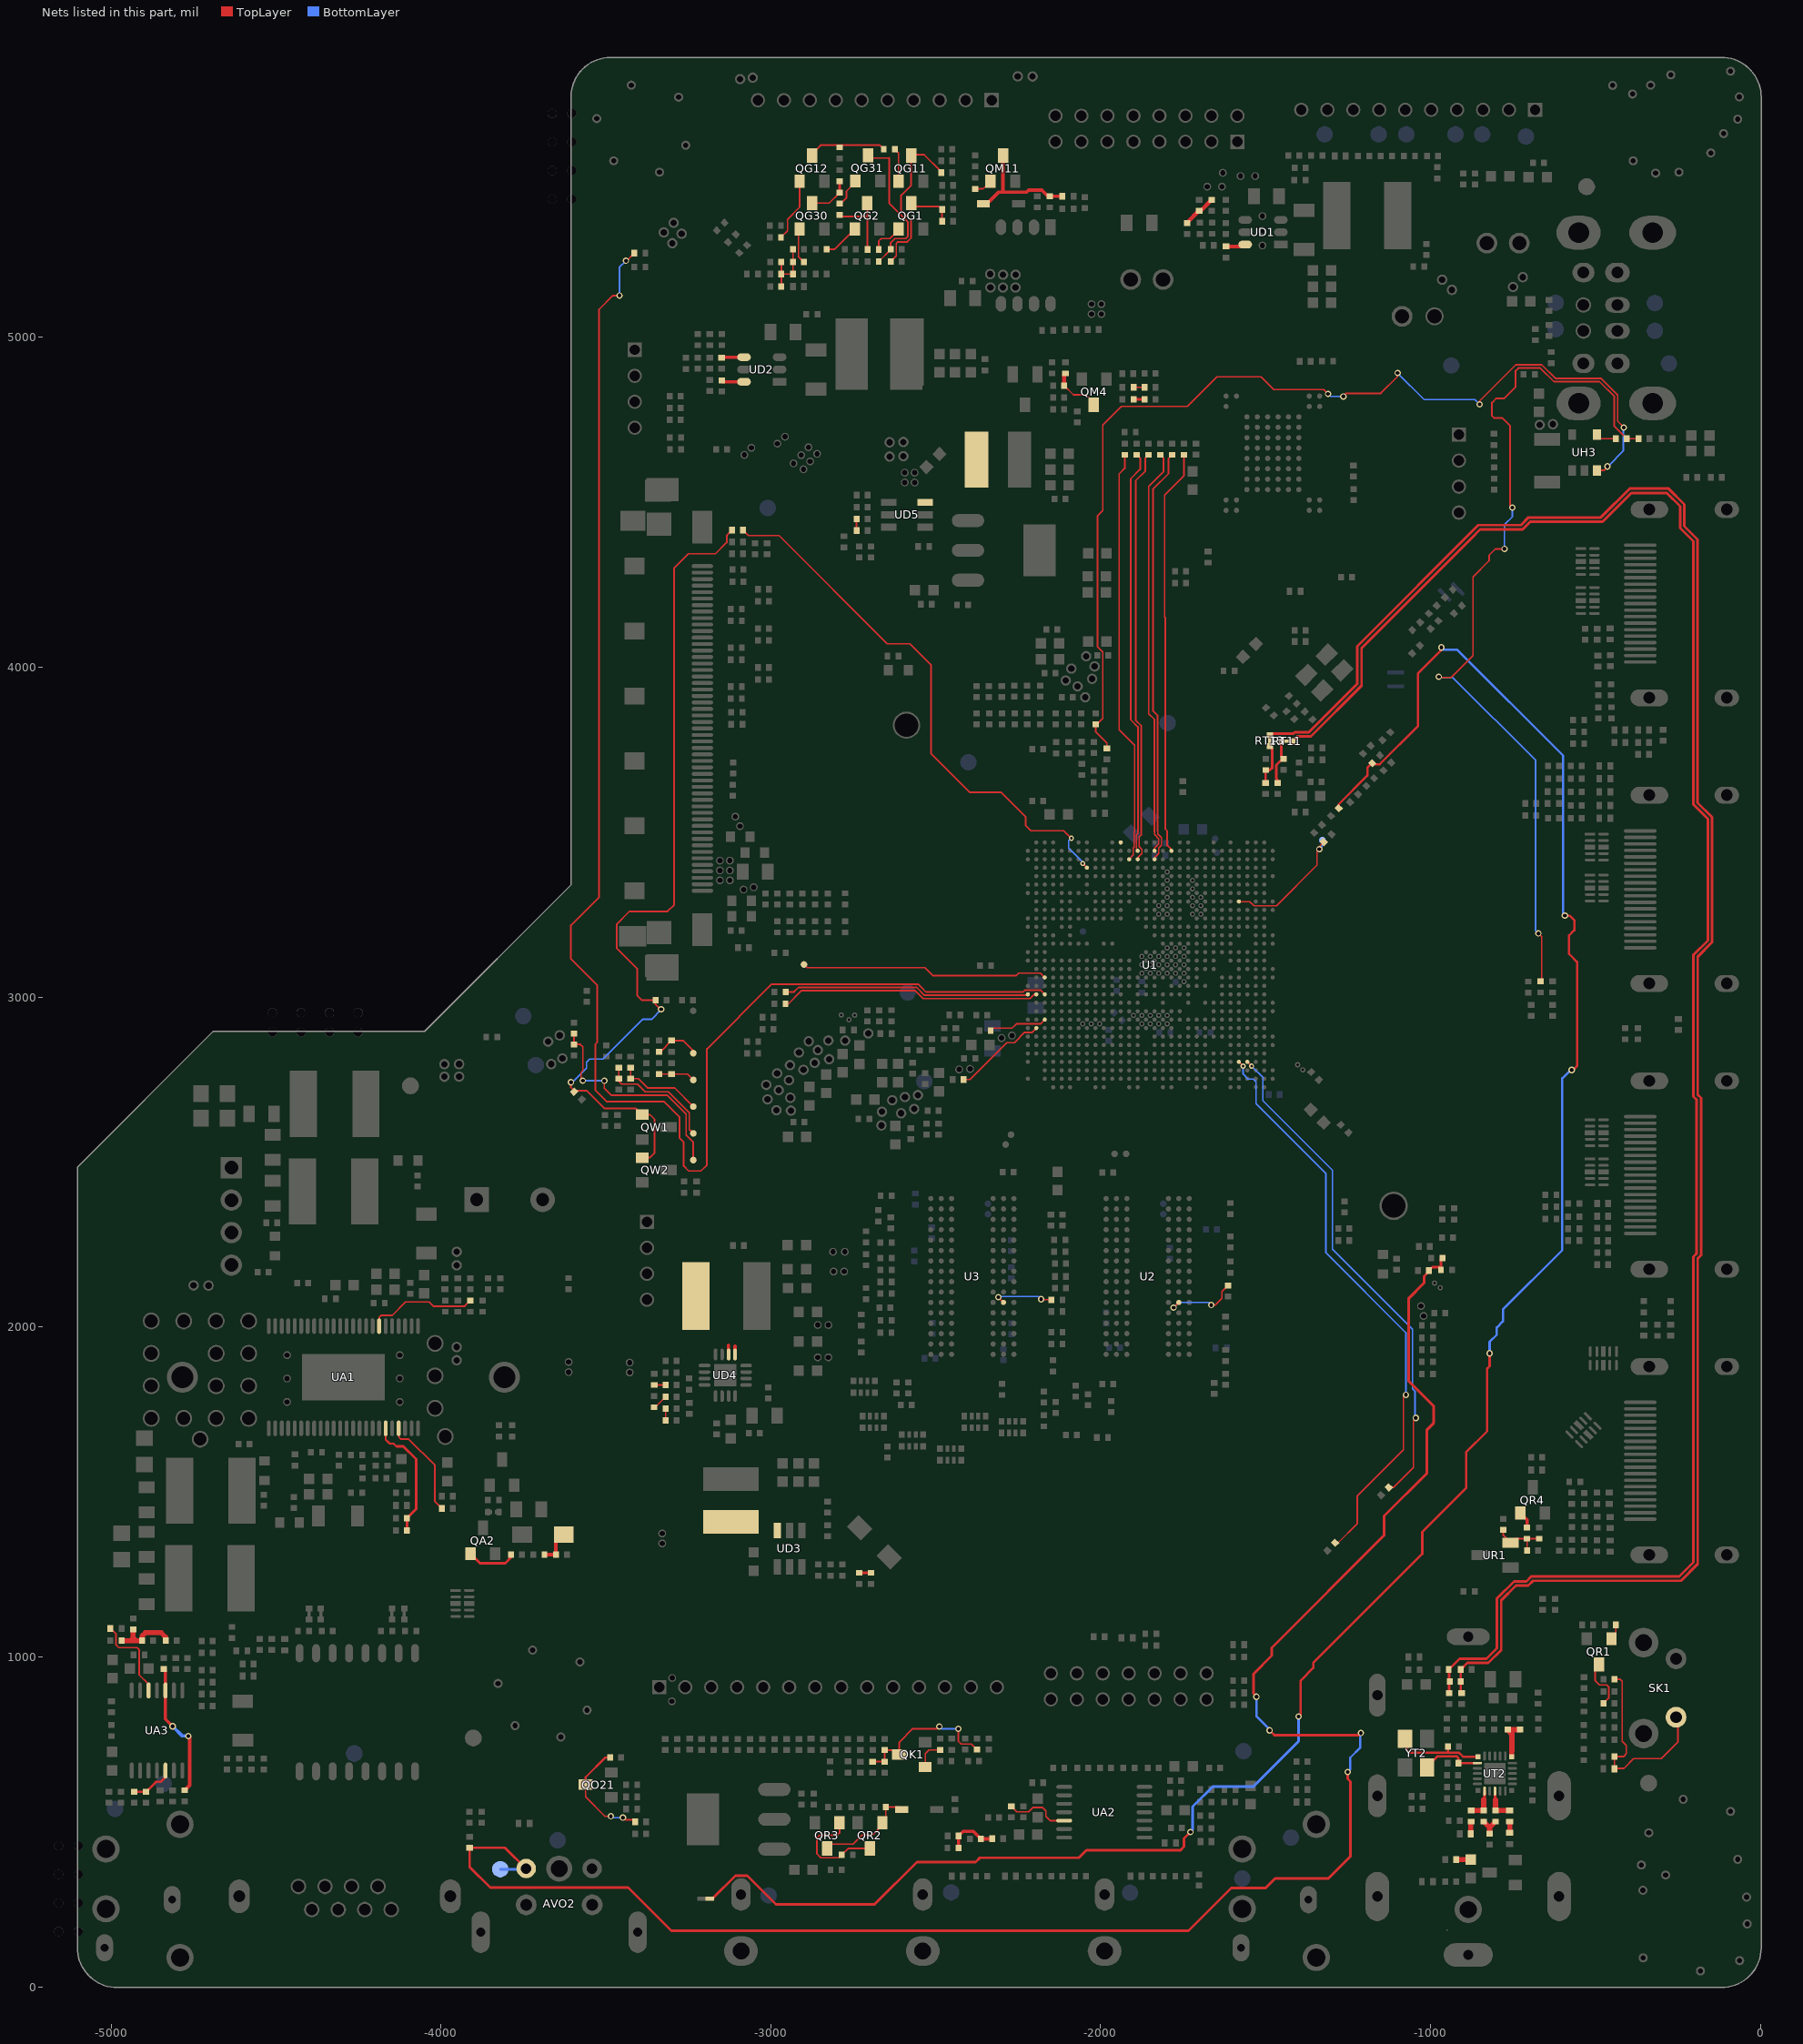
[diagram p0: the nets of this part, all layers, seen from the top]
# Altium PCB MISC86290.PcbDoc (part 26 of 31)
Units mil, origin at the board's own origin, x right, y up, seen from the top; angles counter-clockwise.
Board outline 5104.71 x 5851.49 mil, 2 copper layers (TopLayer, BottomLayer), stack 61.855 mil thick; 1026 components, 667 nets, 4280 pads, 2294 vias.

## Via types
v1: diameter 19.68, hole 11.81, TopLayer to BottomLayer, tented both sides, 1189 vias
v2: diameter 19.68/19.68 (per signal layer), hole 11.81, TopLayer to BottomLayer, tented both sides, 366 vias
v3: diameter 15.75, hole 7.87, TopLayer to BottomLayer, tented both sides, 348 vias
v4: diameter 23.62, hole 15.75, TopLayer to BottomLayer, tented both sides, 309 vias
v5: diameter 15.75/15.75 (per signal layer), hole 7.87, TopLayer to BottomLayer, tented both sides, 59 vias
v6: diameter 24/24 (per signal layer), hole 16, TopLayer to BottomLayer, tented both sides, 23 vias

## Nets (pads, with @x,y where several pads share a name; then routed paths per layer and width w, separated by ;. In a path a pad name is that pad's centre, name@x,y a point inside that pad or via, vN(x,y) a via of type N, cw(c..) or ccw(c..) an arc to the next point about the centre after c; other vN are vias at no path point) (continued)
NetCT6_2: CT6.2 LT10.1 RT10.2 RT11.1 | length 5869.9
  TopLayer w8: RT11.1@-1418.27,3775.82 -1404.32,3789.78 -1403.82,3789.78 ; -1403.82,3790.28 -1363.31,3790.28 -1209.27,3944.31 -1209.27,4058.45 -877.09,4390.63 -851.41,4416.32 -849.72,4418 -720.88,4418 -697.69,4441.2 -478.6,4441.2 -391.3,4528.5 -283.7,4528.5 -243.5,4488.3 -243.5,4422.39 -203.5,4382.39 -203.5,3584.22 -159.5,3540.22 -159.5,3171.74 -203.16,3128.08 -203.16,2698.68 -193.16,2688.68 -193.16,2223.32 -203.16,2213.32 -203.16,1286.87 -246.28,1243.75 -694.78,1243.75 -709.53,1229 -746.68,1229 -798.81,1176.87 -798.81,1026.16 -830.47,994.5 -912.19,994.5 CT6.2@-943.82,962.87 ; CT6.2@-945.08,961.61 CT6.2@-943.82,962.87 ; RT10.2@-943.82,890.34 CT6.2@-943.82,962.87
NetCT9_1: CT9.1 LT6.1 UT2.22 | length 87.5
  TopLayer w7.8: -804.89,568.87 UT2.22@-804.89,593.22
  TopLayer w15.8: CT9.1@-802.89,534.1 LT6.1@-764.9,534.1 ; CT9.1@-802.89,541.1 -802.89,566.26
NetCT9_2: CT9.2 CT23.2 RT3.2 | length 69.4
  TopLayer w15.8: CT23.2@-838.89,500.63 -820.89,482.63 ; RT3.2@-820.89,464.1 -820.89,482.63 ; CT9.2@-802.89,500.63 -820.89,482.63
NetCT12_2: CT12.2 CT27.2 RT11.2 RT11.3 | length 141
  TopLayer w8: CT27.2@-1464,3649.21 -1464,3658.5 -1467.66,3662.16 -1467.66,3703.53 -1448.45,3722.73 CT12.2@-1446.78,3722.73 ; RT11.2@-1452.23,3775.5 -1452.23,3728.18 CT12.2@-1446.78,3722.73 ; CT12.2@-1445.5,3722.73 CT12.2@-1446.78,3722.73
NetCT14_1: CT14.1 CT32.1 RT13.2 RT13.3 | length 126.1
  TopLayer w8: CT32.1@-1500,3649.21 CT14.1@-1500,3685.23 ; CT14.1@-1499.5,3688.5 -1486.88,3688.5 -1480.66,3694.72 -1480.66,3753.66 RT13.2@-1487.5,3760.5
NetCT16_2: CT16.2 CT17.2 UT2.7 | length 121.1
  TopLayer w15: UT2.7@-753.91,697.37 -753.91,713.85
  TopLayer w17: CT16.2@-766.03,779.42 -728.45,779.42 CT17.2@-728.39,779.37 ; CT16.2@-764.39,776.41 -753.89,765.91 -753.89,713.87
NetCT21_1: CT21.1 LT10.2 RT12.2 RT13.1 | length 5932.7
  TopLayer w8: RT13.1@-1483.56,3798.44 -1416.06,3798.44 -1411.72,3802.78 -1369.19,3802.78 -1222.27,3949.7 -1222.27,4063.84 -855.11,4431 -726.27,4431 -703.07,4454.2 -483.99,4454.2 -396.68,4541.5 -278.32,4541.5 -230.5,4493.68 -230.5,4427.78 -190.5,4387.78 -190.5,3589.61 -146.5,3545.61 -146.5,3166.35 -190.16,3122.7 -190.16,2704.07 -180.16,2694.07 -180.16,2217.93 -190.16,2207.93 -190.16,1281.49 -240.9,1230.75 -689.4,1230.75 -704.14,1216 -741.3,1216 -785.81,1171.49 -785.81,1020.77 -825.08,981.5 -888.66,981.5 CT21.1@-908.55,961.61 -908.55,892.8 RT12.2@-905.82,890.07
NetCT23_1: CT23.1 LT5.1 UT2.20 | length 89.1
  TopLayer w7.8: -836.39,568.37 UT2.20@-836.39,593.22
  TopLayer w15.8: LT5.1@-876.89,534.09 CT23.1@-838.89,534.1 ; CT23.1@-838.89,541.1 -838.89,567.37
NetCT24_1: CT24.1 LT9.2 | length 44.1
  TopLayer w15.8: CT24.1@-921.78,385.11 LT9.2@-877.7,385.11
NetCT39_2: CT39.2 UT2.13 YT2.1 | length 278.5
  TopLayer w7: YT2.1@-1072.46,753.31 -1072.46,718.46 -1064.07,710.07 -947.65,710.07 ; CT39.2@-947.65,728.42 -947.65,710.07 ; UT2.13@-855.89,697.35 -901.66,697.35 -914.38,710.07 -947.65,710.07
NetCT40_2: CT40.2 UT2.14 YT2.3 | length 204.1
  TopLayer w7: YT2.3@-1018.54,649.19 -1018.54,659.08 -979.54,698.07 -920.24,698.07 -915.65,693.48 CT40.2@-915.65,677.86 UT2.14@-858.04,677.86
NetCVBSOUT1_1: CVBSOUT1.1 R41.2 U1.AC5 | length 401.1
  TopLayer w3.94: U1.AC5@-1581.02,3289.96 -1547.71,3289.96 -1534.78,3277.02 -1472.5,3277.02
  TopLayer w5: -1472.5,3277.17 -1467.58,3277.17 -1344.5,3400.25 v1@-1344.5,3448.56 ; v1(-1337.16,3448.56) -1337.16,3456.84 R41.2@-1323.83,3470.17
  BottomLayer w5: v1(-1337.16,3448.56) -1329,3456.72 CVBSOUT1.1@-1329,3478
NetDA9_A: DA9.A RA22.2 RA26.2 | length 104.1
  TopLayer w10: RA26.2@-3686.27,1310 RA22.2@-3651.73,1310 -3651.73,1350.28 DA9.A@-3631.01,1371
NetDM11_A: DM11.A QM11.C RM13.2 RM14.1 | length 366.9
  TopLayer w5: DM11.A@-2371.28,5405 DM11.A@-2355.4,5405
  TopLayer w10: DM11.A@-2336.42,5413.4 -2309,5440.83 -2224.17,5440.83 -2218.41,5446.59 -2178.26,5446.59 -2159.67,5428 RM13.2@-2115.98,5428 ; -2296.25,5442.07 QM11.C@-2296.25,5551.16
NetDR2_K: DR2.K RR9.1 RR10.2 SK1.2 | length 627.4
  TopLayer w5: RR9.1@-442.27,932 -425,932 -419,926 -419,744.5 -406.5,732 -406.5,706.29 -415.29,697.5 RR10.2@-442.77,697.5 -442.77,661.73 -414.27,661.73 -384.5,691.5 -300,691.5 -250.43,741.07 SK1.2@-250.43,816.93
NetDR3_A: DR3.A QR2.B QR3.C RR15.1 | length 316.5
  TopLayer w5: QR3.C@-2829.75,418.97 -2816.22,432.5 -2750.5,432.5 -2723,460 -2692,460 -2651.25,500.75 RR15.1@-2651.25,544.99 -2611.14,544.99 DR3.A@-2603.15,537 ; RR15.1@-2650.24,546 -2651.25,547 RR15.1@-2646.25,552
NetEJ_TCK_1: EJ_TCK.1 R144.1 R147.2 | length 362.8
  TopLayer w5: R147.2@-3461,2786.27 R144.1@-3461,2752.84 -3461,2745 -3452.38,2736.38 -3404.38,2736.38 -3380.91,2712.91 -3310.63,2712.91 -3247,2649.28 -3247,2598 -3236,2587 EJ_TCK.1@-3235,2587
NetEJ_TDI_1: EJ_TDI.1 R145.1 R149.2 | length 258.6
  TopLayer w5: R149.2@-3425,2786.27 R145.1@-3425,2752.73 -3401.73,2752.73 -3374,2725 -3292,2725 EJ_TDI.1@-3235,2668
NetEJ_TDO_1: EJ_TDO.1 R148.2 R207.1 | length 111.4
  TopLayer w5: R148.2@-3339,2766.77 R207.1@-3301,2766.77 -3252.77,2766.77 EJ_TDO.1@-3235,2749
NetEJ_TMS_1: EJ_TMS.1 R146.2 R206.1 | length 137.8
  TopLayer w5: R146.2@-3339,2834.77 -3334.46,2834.77 R206.1@-3301,2868.23 -3266.23,2868.23 -3235,2837 EJ_TMS.1@-3235,2830
NetI2S_IN_MCK_1: I2S_IN_MCK.1 U1.P28 | length 750.7
  TopLayer w3.94: -2250.95,3070.48 -2248.99,3072.44 -2182.4,3072.44 U1.P28@-2169.61,3059.65
  TopLayer w5: I2S_IN_MCK.1@-2899.5,3099 -2889.84,3089.34 -2532.86,3089.34 -2509.05,3065.53 ; -2507.8,3065.53 -2255.9,3065.53 -2250.95,3070.48
NetLD21_1: LD21.1 UD3.3
NetLD31_1: LD31.1 UD4.1 UD4.2 | length 54
  TopLayer w10: UD4.2@-3128.17,1916.68 -3128.17,1945.08 ; UD4.1@-3108.48,1916.68 -3108.48,1942.27
NetLD51_1: LD51.1 UD5.3
NetLT3_1: LT3.1 LT5.2 | length 25.1
  TopLayer w15.8: -878.17,474.3 LT5.2@-878.17,499.36
NetLT6_2: LT6.2 LT7.1 | length 32.7
  TopLayer w15: LT7.1@-760.22,466.24 LT6.2@-760.22,498.95
NetQA2_B: QA2.B RA24.1 | length 150.4
  TopLayer w8: QA2.B@-3910.5,1313 -3881.66,1284.16 -3805,1284.16 -3787.73,1301.43 RA24.1@-3787.73,1310
NetQG1_B: QG1.B RG8.1 | length 102.6
  TopLayer w5: RG8.1@-2672.77,5266.5 -2672.77,5292.73 -2665.59,5299.91 -2639.59,5299.91 -2612.75,5326.75 QG1.B@-2612.75,5329
NetQG1_C: QG1.C RG1.1 RG3.2 | length 138
  TopLayer w5: QG1.C@-2574.75,5408.03 -2563.72,5397 -2490.14,5397 RG3.2@-2480.98,5387.84 RG1.1@-2480.98,5352
NetQG2_B: QG2.B RG2.1 | length 110.1
  TopLayer w5: RG2.1@-2830.27,5267 -2807,5267 -2747.14,5326.86 QG2.B@-2747.14,5329
NetQG2_C: QG2.C RG7.1 RG8.2 | length 211.9
  TopLayer w5: -2781.16,5366.31 -2708.5,5366.31 ; RG8.2@-2707.5,5267.77 QG2.C@-2707.5,5407.03
NetQG11_B: QG11.B RG18.1 | length 99.6
  TopLayer w5: RG18.1@-2624.27,5571 -2612.75,5559.48 QG11.B@-2612.75,5476.12
NetQG11_C: QG11.C RG12.1 RG13.1 | length 502.6
  TopLayer w5: RG12.1@-2636.73,5230.5 -2620,5247.23 -2620,5285 -2615.5,5289.5 -2586.36,5289.5 -2575,5300.86 -2575,5354.5 -2605,5384.5 -2605,5431 -2574.75,5461.25 QG11.C@-2574.75,5551.16 -2574.75,5554.16 -2535.16,5554.16 -2486,5505 RG13.1@-2483.73,5505
NetQG12_B: QG12.B RG11.1 | length 193
  TopLayer w5: RG11.1@-2969.27,5303.5 -2949.5,5323.27 -2949.5,5358.09 -2912.81,5394.77 QG12.B@-2912.81,5473.12
NetQG12_C: QG12.C RG17.1 RG18.2 | length 238.6
  TopLayer w5: QG12.C@-2874.81,5551.16 -2874.81,5557.07 -2849.04,5582.85 -2669.58,5582.85 RG18.2@-2657.73,5571
NetQG30_B: QG30.B RG34.1 | length 104.7
  TopLayer w5: QG30.B@-2916.02,5325.79 -2916.02,5244.76 RG34.1@-2899.27,5228
NetQG30_C: QG30.C RG36.2 RG38.1 | length 131.7
  TopLayer w5: QG30.C@-2874.81,5407.03 -2823.2,5407.03 RG36.2@-2791,5439.23
  TopLayer w8: RG36.2@-2791,5439.23 RG38.1@-2791,5473.77
NetQG31_B: QG31.B RG36.1 | length 92.6
  TopLayer w5: RG36.1@-2791,5405.77 -2788.05,5405.77 -2771,5422.82 -2771,5442.47 -2743.5,5469.97 QG31.B@-2743.5,5474 QG31.B@-2743.5,5477
NetQG31_C: QG31.C RG37.1 RG39.1 | length 462.7
  TopLayer w5: QG31.C@-2705.5,5555.03 -2694.47,5544 -2642.02,5544 -2641,5545.02 -2641,5406.36 -2585,5350.36 -2585,5305 -2590.5,5299.5 -2624,5299.5 -2636.73,5286.77 RG37.1@-2636.73,5267 ; RG39.1@-2672.77,5230 RG37.1@-2636.73,5266.04
NetQK1_B: QK1.B RK15.1 | length 96.5
  TopLayer w5: QK1.B@-2532.5,666 -2531.5,667 -2531.5,706.5 -2520.5,717.5 -2487.77,717.5 RK15.1@-2487,718.27 ; RK15.1@-2487.47,717.53 RK15.1@-2481.25,717.53
NetQK1_C: QK1.C RK10.1 RK37.2 RK38.2 RK42.1 | length 455.8
  TopLayer w5: RK42.1@-2691.5,682.23 RK10.1@-2655.5,682.23 ; RK10.1@-2655,681.73 RK37.2@-2655,717.27 -2623.8,717.27 QK1.C@-2610.53,704 -2610.53,741.16 -2569.68,782.02 v1@-2495.48,782.02 ; v1(-2431.5,782.02) -2431.5,743.92 -2423.08,735.5 -2391.73,735.5 RK38.2@-2375,718.77
  BottomLayer w5: v1(-2489,788.5) -2482.52,782.02 v1(-2431.5,782.02)
NetQM4_C: QM4.C RM2.2 RM3.1 | length 156.4
  TopLayer w5: RM3.1@-2110.77,4854 -2082.77,4826 -2044,4826 -2020.75,4802.75 QM4.C@-2020.75,4795.97
  TopLayer w12: RM3.1@-2110.77,4854 -2110.77,4887.04 RM2.2@-2107,4890.81
NetQM11_B: QM11.B RM11.2 | length 56
  TopLayer w5: RM11.2@-2380.81,5450.39 -2356.99,5450.39 QM11.B@-2334.25,5473.13
NetQO21_C: QO21.C RO22.1 RO23.2 | length 331
  TopLayer w5: QO21.C@-3561.53,612.5 -3561.53,575.2 -3502.94,516.6 ; -3502.59,516.96 -3502.23,516.6 v1(-3484.92,516.69) v1(-3484.92,516.69) ; v1@-3442,506 -3417.46,506 RO23.2@-3411.46,500
  TopLayer w6: QO21.C@-3561.53,612.5 -3561.53,634.93 -3501.46,695 RO22.1@-3487,695
  BottomLayer w5: v1(-3484.92,516.69) -3480.73,512.5 v1(-3448.5,512.5)
NetQR1_B: QR1.B RR4.2 | length 52.5
  TopLayer w5: QR1.B@-451.5,1055 -438.27,1068.23 RR4.2@-438.27,1097 RR4.2@-438.27,1102
NetQR1_C: QR1.C RR5.2 | length 159.2
  TopLayer w5: QR1.C@-489.5,976.97 -500.8,965.67 -500.8,927.76 -487.7,914.66 -465.92,914.66 -459.37,908.11 -459.37,876.5 -475.73,860.14 RR5.2@-475.73,859.16
NetQR2_C: QR2.C QR3.B RR16.2 | length 331.1
  TopLayer w5: QR3.B@-2791.75,497 -2791.75,466.25 -2799,459 -2853,459 -2860,452 -2860,402.63 -2848.19,390.81 -2794.17,390.81 RR16.2@-2784.98,400 -2766.01,418.97 QR2.C@-2699.75,418.97
NetQR4_B: QR4.B RR1.1 | length 52.8
  TopLayer w10: QR4.B@-728.1,1436 -707.5,1415.4 RR1.1@-707.5,1391.73
NetQW1_G: QW1.G QW2.G RW1.1 RW4.2 RW5.2 | length 2627.6
  TopLayer w5: v1(-3606,2742) -3606,2726 -3596,2716 -3557.64,2716 -3504.55,2662.91 -3409.41,2662.91 QW1.G@-3390,2643.5 -3366.5,2643.5 -3352.5,2629.5 -3352.5,2528 -3367,2513.5 QW2.G@-3390,2513.5 ; v1(-3332.5,2963.5) -3334,2962 -3349.73,2977.73 RW1.1@-3349.73,2991 -3391.71,2991 -3404.71,3004 -3404.71,3085 -3466.85,3147.13 -3466.85,3221.58 -3428.43,3260 -3312.88,3260 -3293.21,3279.66 -3293.21,4301.04 -3250.25,4344 -3167.86,4344 -3133.78,4378.07 -3133.78,4399.66 RW5.2@-3117.44,4416
  BottomLayer w5: v1(-3606,2742) -3601.33,2742 -3559,2784.33 -3559,2802.37 -3549.35,2812.01 -3509.23,2812.01 -3388.59,2932.66 -3361.84,2932.66 -3332.5,2962 v1(-3332.5,2963.5)
NetR39_1: R39.1 RI115.2 RI116.JP_2K | length 6588.3
  TopLayer w7: v1@-1393.82,825.18 -1393.82,927.91 -1355.49,966.24 -1355.49,982.23 -1025.09,1312.63 -1025.09,1378.94 -892.28,1511.74 -892.28,1620.42 -828.34,1684.36 -828.34,1874.51 -821,1881.85 v1(-821,1920) ; R39.1@-1278.17,3572.83 -1278.17,3584.77 -1191.5,3671.44 -1191.5,3696 -1178.33,3709.17 RI115.2@-1176.83,3709.17 -1173.66,3706 -1154,3706 -1038,3822 -1038,3982.02 v1@-967,4053.02 ; v1(-593,3247) -578,3247 -564,3233 -564,3203 -580.34,3186.66 -580.34,3131.49 -556,3107.15 -556,2791 v1@-568,2779
  TopLayer w8: RI116.JP_2K@-3175.25,267 -3175.25,268.84 -3107.35,336.74 -3071.74,336.74 -2984.5,249.5 -2685.95,249.5 -2557.3,378.16 -2378.84,378.16 -2366.16,390.84 -2066.32,390.84 -2043.16,414 -1758,414 -1747.57,424.43 -1747.57,449.43 v1(-1728,469)
  BottomLayer w7: v1@-965.66,4053.66 -919.78,4053.66 -598,3731.88 v1@-598,3252 ; v1(-821,1920) -821,1955 -799.34,1976.66 -799.34,1998.54 -780.54,2017.34 -780.54,2053.54 -601,2233.09 -601,2753.94 v1@-575.94,2779
  BottomLayer w8: v1(-1728,469) -1721.04,475.96 -1721.04,545.96 -1660,607 -1537.31,607 -1400.16,744.15 v1@-1400.16,818.84
  other v1: -1400,819 -572,2779 -967,4060
NetR48_2: R48.2 U1.H29 | length 285.2
  TopLayer w5: R48.2@-2415.72,2750.03 -2396.72,2750.03 -2284.72,2862.03 -2261.72,2862.03 -2230.45,2893.31 -2207.99,2893.31 U1.H29@-2195.2,2906.1
NetR49_2: R49.2 U1.J28 | length 178.1
  TopLayer w5: R49.2@-2333.72,2898.03 -2325.72,2906.03 -2268.76,2906.03 -2255.9,2918.9 -2182.4,2918.9 U1.J28@-2169.61,2931.69
NetR64_2: R64.2 U2.L8 | length 233.7
  TopLayer w3.94: v2(-1778.86,2058.66) U2.L8@-1763.11,2074.41 ; v2(-1664.69,2066.54) -1652.87,2066.54 -1632.2,2087.2 -1632.2,2107.2 R64.2@-1613.5,2125.91
  BottomLayer w3.94: v2(-1778.86,2058.66) -1763.11,2074.41 -1672.56,2074.41 v2(-1664.69,2066.54)
NetR100_2: R100.2 U3.L8 | length 188.3
  TopLayer w3.94: v2(-2310.35,2090.16) U3.L8@-2294.61,2074.41 ; v2(-2180.43,2084.25) -2178.46,2082.28 R100.2@-2149.25,2082.28
  BottomLayer w3.94: v2(-2310.35,2090.16) -2308.39,2092.13 -2188.31,2092.13 v2(-2180.43,2084.25)
NetR120_1: R120.1 R121.2 | length 36
  TopLayer w8: R120.1@-2732.16,1254.73 R121.2@-2696.16,1254.73
NetR125_1: R125.1 U1.M28 | length 4665.2
  TopLayer w5: -3606.16,3217.29 -3606.16,3115.88 -3526,3035.72 -3526,2863 -3532.01,2856.99 -3532.01,2718.65 -3496.27,2682.91 -3323.05,2682.91 -3277,2636.86 -3277,2573.29 -3264,2560.29 -3264,2487.86 -3249.14,2473 -3212,2473 -3193.91,2491.09 -3193.91,2842.86 -2997.42,3039.34 -2553.86,3039.34 -2542.76,3028.24 -2530,3015.53 ; -3606.16,3218 -3520.61,3303.55 -3520.61,5085.21 -3478.82,5127 v1(-3459,5127) ; v1(-3439,5232.5) -3436.73,5232.5 R125.1@-3413.73,5255.5 ; -2528.75,3015.53 -2234.95,3015.53 -2229.22,3021.26 -2182.4,3021.26 U1.M28@-2169.61,3008.46
  BottomLayer w5: v1(-3459,5127) -3459,5212.5 v1(-3439,5232.5)
NetR135_1: R135.1 U1.D5 | length 1771.9
  TopLayer w4.92: U1.D5@-1581.02,2803.74 v3(-1568.23,2790.94)
  TopLayer w5: R135.1@-1289.17,1345.83 -1280.11,1345.83 -1222.01,1403.94 -1222.01,1488.34 -1082.22,1628.13 -1082.22,1787.85 -1075.3,1794.78 v1(-1074.88,1794.36)
  BottomLayer w3.94: -1568.23,2766.54 -1553.27,2751.57 -1536.87,2751.57 -1528.91,2743.62
  BottomLayer w4.92: -1568.23,2766.54 v3(-1568.23,2790.94)
  BottomLayer w5: -1529.19,2743.35 -1529.19,2677.49 -1317.67,2465.98 -1317.67,2225.69 -1074.88,1982.91 v1(-1074.88,1794.36)
NetR136_1: R136.1 U1.D4 | length 1543.8
  TopLayer w4.92: U1.D4@-1555.43,2803.74 v3(-1542.64,2790.94) ; R136.1@-1126.67,1513.83 -1112.17,1513.83 -1052.26,1573.74 -1052.26,1716.8 v1(-1044.88,1724.18)
  BottomLayer w4.92: v3(-1542.64,2790.94) -1508.67,2756.98 -1508.67,2686.03 -1297.67,2475.03 -1297.67,2235.67 -1054.92,1992.92 -1054.92,1812.42 -1047,1804.5 -1047,1726.3 v1(-1044.88,1724.18)
NetR143_1: R143.1 R150.2 SOC_RESETn.1 | length 698.1
  TopLayer w5: R143.1@-3597,2889.27 R150.2@-3597,2856.73 -3577.73,2856.73 -3570,2849 -3570,2777 -3575.5,2771.5 -3575.5,2746.5 v1(-3570,2746.5) ; v1(-3504.67,2746.41) -3505,2746.07 -3505,2723.5 -3484.41,2702.91 -3314.77,2702.91 -3257,2645.14 -3257,2581.57 -3235,2559.57 SOC_RESETn.1@-3235,2506 SOC_RESETn.1@-3227,2506
  BottomLayer w5: v1(-3570,2746.5) v1(-3570,2746.5) v1(-3504.67,2746.41)
NetR200_2: R200.2 U1.M29 | length 788.4
  TopLayer w5: R200.2@-2951.37,2975.37 -2907.4,3019.34 -2562.19,3019.34 -2538.38,2995.53 ; -2537.13,2995.53 -2214.42,2995.53 -2201.49,3008.46 U1.M29@-2195.2,3008.46
NetR201_2: R201.2 U1.M30 | length 749.8
  TopLayer w5: R201.2@-2955.27,3016 -2929.5,3016 -2916.16,3029.34 -2558,3029.34 -2534.19,3005.53 ; -2532.94,3005.53 -2223.72,3005.53 U1.M30@-2220.79,3008.46
NetRA5_2: RA5.2 RA7.1 UA1.19 | length 378.9
  TopLayer w6: UA1.19@-4167.8,1688.79 -4167.8,1659.04 -4155.22,1646.46 -4143.59,1646.46 -4136.13,1639 -4134.22,1639
  TopLayer w8: UA1.19@-4167.8,1688.79 UA1.19@-4167.8,1692.73 ; -4134.22,1638.5 -4114.4,1638.5 -4075,1599.1 -4075,1448.27 RA5.2@-4103.27,1420 RA7.1@-4103.27,1383
NetRA15_1: RA15.1 UA1.21 | length 314.3
  TopLayer w5: UA1.21@-4128.43,1692.73 -4128.43,1667.43 -4121,1660 -4097.97,1660 -4018.5,1580.53 -4018.5,1470.77 RA15.1@-3997.73,1450
  TopLayer w6: UA1.21@-4128.43,1688.79 UA1.21@-4128.43,1692.73
NetRA21_2: RA21.2 UA1.31 | length 334.8
  TopLayer w5: UA1.31@-4187.48,2002.77 -4187.48,2029.52 -4182,2035 -4148.32,2035 -4107.32,2076 -4036,2076 -4023,2063 -3927.73,2063 RA21.2@-3911,2079.73
NetRD3_1: RD3.1 UD1.6 | length 62.3
  TopLayer w12: RD3.1@-1620.25,5275.73 -1567.83,5275.73 UD1.6@-1562.04,5281.51 ; UD1.6@-1575.73,5281.51 UD1.6@-1574.52,5282.73
NetRD4_2: RD4.2 RD5.2 RD6.2 | length 110.3
  TopLayer w12: RD5.2@-1737.47,5346.73 -1737.47,5349.04 RD6.2@-1701.25,5385.27 ; RD6.2@-1696.51,5385.27 RD6.2@-1701.25,5385.27 ; RD4.2@-1664.14,5417.63 -1664.04,5417.73 RD4.2@-1663.25,5417.73 ; RD4.2@-1663.25,5416.73 -1664.04,5416.73 -1695.51,5385.27 RD6.2@-1701.25,5385.27
NetRD13_1: RD13.1 UD2.6 | length 66.7
  TopLayer w10: RD13.1@-3148.25,4865.45 UD2.6@-3081.55,4865.45
NetRD14_1: RD14.1 UD2.4 | length 67.7
  TopLayer w10: RD14.1@-3149.25,4940.26 UD2.4@-3081.55,4940.26
NetRD32_2: RD32.2 RD33.2 | length 36
  TopLayer w5: RD33.2@-3318.73,1717 RD32.2@-3318.73,1753
NetRD34_2: RD34.2 RD35.2 | length 34
  TopLayer w5: RD35.2@-3353.5,1824.27 RD34.2@-3319.46,1824.27
NetRD36_2: RD36.2 RD37.2 | length 44.9
  TopLayer w5: RD37.2@-3350.96,1756.77 RD36.2@-3319.23,1788.5
NetRD54_1: RD54.1 RD55.2 | length 35.2
  TopLayer w5: RD54.1@-2740.17,4414.58 RD55.2@-2740.17,4449.79
NetRD57_1: RD57.1 RD59.2 | length 33.5
  TopLayer w8: RD57.1@-1900.52,4811.95 RD59.2@-1866.98,4811.95
NetRD58_2: RD58.2 RF56.1 | length 33.8
  TopLayer w5: RF56.1@-1900.52,4848.95 RD58.2@-1866.71,4848.95
NetRF3_1: RF3.1 U1.AH15 | length 1268.9
  TopLayer w3.94: U1.AH15@-1836.93,3417.91 -1836.93,3422.83 -1836.4,3423.33 -1824.13,3435.59 -1824.13,3452.36 -1816.26,3460.24 -1816.26,3483.86 -1827.22,3494.82 -1827.22,3503.03
  TopLayer w5: -1827.22,3503.03 -1827.22,3853.57 -1841,3867.34 -1841,4540.76 -1794.25,4587.51 -1794.25,4633.11 RF3.1@-1783.25,4644.11
NetRF4_1: RF4.1 U1.AJ15 | length 1241.2
  TopLayer w3.94: -1837.22,3500.47 -1837.22,3493.01 -1824.13,3479.92 -1824.13,3464.17 -1836.93,3451.38 U1.AJ15@-1836.93,3443.5
  TopLayer w5: -1837.22,3500.47 -1837.22,3842.33 -1854.25,3859.35 -1854.25,4548.73 -1809.25,4593.73 -1809.25,4634.11 RF4.1@-1819.25,4644.11
NetRF5_1: RF5.1 U1.AJ17 | length 1221.4
  TopLayer w3.94: U1.AJ17@-1888.11,3443.5 -1891.06,3446.46 -1891.06,3491.69 -1887.22,3495.53 -1887.22,3499.61
  TopLayer w5: -1887.22,3499.61 -1887.22,3819.13 -1908.95,3840.86 -1908.95,4571.62 -1880.25,4600.32 -1880.25,4634.11 RF5.1@-1885.25,4639.11
NetRF6_1: RF6.1 U1.AJ13 | length 1233.3
  TopLayer w3.94: -1792.64,3454.33 -1785.75,3447.44 U1.AJ13@-1785.75,3443.5
  TopLayer w5: -1792.64,3454.33 -1798.22,3459.92 -1798.22,3503.75 -1803.75,3509.27 -1803.75,4150.25 -1806,4152.5 -1806,4522.36 -1747.25,4581.11 RF6.1@-1747.25,4644.11
NetRF7_1: RF7.1 U1.AH17 | length 1260.6
  TopLayer w3.94: U1.AH17@-1888.11,3417.91 -1887.94,3422.92 -1874.69,3436.17 -1874.69,3447.67 -1883.19,3456.17 -1883.19,3485.83 -1877.22,3491.79 -1877.22,3496.22
  TopLayer w5: -1877.22,3496.22 -1877.22,3823.28 -1893.95,3840.01 -1893.95,4565.4 -1865.25,4594.11 -1865.25,4634.11 RF7.1@-1855.25,4644.11
NetRF8_1: RF8.1 U1.AH18 | length 1259.3
  TopLayer w3.94: U1.AH18@-1913.7,3417.91 -1900.91,3430.71 -1900.91,3452.36 -1898.94,3454.33 -1898.94,3499.86 -1897.22,3501.57
  TopLayer w5: RF8.1@-1927.25,4644.11 -1927.25,4602.82 -1943.95,4586.11 -1943.95,3809.95 -1897.22,3763.22 -1897.22,3501.57
NetRG30_1: RG30.1 RG31.2 RG32.2 RG33.2 RG34.2 RG35.2 | length 185.5
  TopLayer w5: RG32.2@-2968.27,5154 RG33.2@-2968.27,5192 ; RG30.1@-2968.27,5229 RG33.2@-2968.27,5192 ; RG35.2@-2932.73,5267 RG34.2@-2932.73,5229 RG31.2@-2932.73,5192 RG33.2@-2968.27,5192
NetRO19_1: RO19.1 RO20.2 RO21.1 RO46.1 | length 188.7
  TopLayer w10: RO46.1@-2431.27,421 -2431.27,456.73 RO19.1@-2431,457 -2417.16,470.84 -2385.84,470.84 RO20.2@-2363,448 ; RO20.2@-2363,448 -2329.73,448 RO21.1@-2328.73,449 -2362,449 RO20.2@-2363,448
NetRO29_2: RO29.2 UA2.5 | length 199.1
  TopLayer w5: RO29.2@-2271,546.73 -2254.27,530 -2219,530 -2206,543 -2176,543 -2166,533 -2166,516 -2153.41,503.41 UA2.5@-2110.55,503.41
NetRO33_2: RO33.2 RO37.1 UA3.3 | length 433.8
  TopLayer w10: RO33.2@-4837.84,961.5 -4835.32,958.98 UA3.3@-4835.32,898.32 ; UA3.3@-4835.32,878.32 UA3.3@-4835.32,898.32 ; v1(-4813.5,789.5) -4835.32,811.32 UA3.3@-4835.32,898.32 ; RO37.1@-4777,595.73 -4762,610.73 -4762,755.75 v1(-4766.25,760)
  BottomLayer w10: v1(-4813.5,789.5) -4784,760 v1(-4766.25,760)
NetRO34_2: RO34.2 RO38.1 UA3.12 | length 133
  TopLayer w7: RO38.1@-4930.5,590.73 RO34.2@-4894.5,590.73 -4894.21,590.73 -4863.94,621 -4850.5,621 -4835.32,636.18 UA3.12@-4835.32,655.21
NetRO41_1: RO41.1 RO42.1 RO43.2 RO47.1 | length 217.2
  TopLayer w15: RO42.1@-4968.43,1049 -4941,1049 ; RO47.1@-4933,1083.27 -4933,1057 ; RO41.1@-4834.25,1049 -4834.25,1059.25 -4848,1073 -4896,1073 -4905.98,1063.02 RO43.2@-4905.98,1049 -4925,1049 ; -4941,1049 -4925,1049 ; -4941,1049 -4933,1057 ; -4933,1057 -4925,1049
NetRO44_2: RO44.2 UA3.5 | length 268.3
  TopLayer w5: RO44.2@-5001.89,1086 -4985,1069.11 -4985,1036 -4977,1028 -4921,1028 -4915,1022 -4915,946 -4886.51,917.51 UA3.5@-4886.51,898.32
NetRR1_2: RR1.2 RR2.1 RR18.1 RR19.1 UR1.2 | length 157.5
  TopLayer w5: RR2.1@-779.5,1384.54 -779.5,1368.15 UR1.2@-757.26,1345.9 ; UR1.2@-744.89,1358.27 RR1.2@-707.5,1358.27 ; RR19.1@-707.5,1322.5 RR1.2@-707.5,1358.27 ; RR18.1@-671,1358.27 RR1.2@-707.5,1358.27
NetRU3_1: RU3.1 RU6.1 RU10.1 | length 2743.2
  TopLayer w5: v1@-976,3978 -967.34,3969.34 -937.31,3969.34 -871.5,4035.15 -871.5,4273.97 -822.66,4322.82 -822.66,4339.34 -803,4359 v1(-776,4359) ; v1(-752,4484) -758.66,4490.66 -758.66,4731.79 -782.87,4756 -808,4756 -814,4762 -814,4802.46 -801.7,4814.76 -777.24,4814.76 -742,4850 -742,4899 -734,4907 -667.14,4907 -626.14,4866 -488,4866 -443,4821 -443,4730.73 RU6.1@-405.27,4693 RU3.1@-369.73,4693 ; v1(-673,3193) -663,3183 RU10.1@-663,3050.68
  BottomLayer w5: v1@-976,3978 -967.34,3969.34 -933.04,3969.34 -681.34,3717.64 -681.34,3201.34 v1(-673,3193) ; v1(-776,4359) -776,4432 -752,4456 v1(-752,4484)
  other v1: -975,3971
NetRU5_2: RU5.2 RU9.2 UH3.3 | length 3115.5
  TopLayer w5: RU9.2@-1981.5,3754.23 -1981.5,3770 -2015,3803.5 RU5.2@-2015,3827.27 -2012.05,3827.27 -1993.95,3845.36 -1993.95,4046.52 -2010,4062.57 -2010,4458.95 -1993.95,4475 -1993.95,4734.54 -1937.5,4791 -1737.24,4791 -1647.75,4880.49 -1513.82,4880.49 -1475.33,4842 -1324,4842 v1(-1311,4829) ; v1(-1264.5,4821) -1264.5,4822 -1255.87,4830.63 -1150.7,4830.63 -1100,4881.32 v1(-1100,4892) ; v1(-851.34,4797.16) -851.34,4807.54 -741.88,4917 -663,4917 -622,4876 -483.86,4876 -433,4825.14 -433,4746 v1(-414,4727) ; UH3.3@-495.6,4596.87 -474.66,4596.87 v1@-460.87,4610.66
  BottomLayer w5: v1(-1311,4829) -1303,4821 v1(-1264.5,4821) ; v1(-1100,4892) -1019.5,4811.5 -865.68,4811.5 v1(-851.34,4797.16) ; v1@-460.87,4610.66 -416,4655.53 -416,4725 v1(-414,4727)
  other v1: -464,4609
NetRU6_2: RU6.2 UH3.4 | length 61.9
  TopLayer w5: UH3.4@-495.6,4705.13 -483.46,4693 RU6.2@-438.73,4693
OPTICAL: AVO2.1 CO1.1 DO2.K OPTICAL.1 RO1.2 RO2.2 | length 5622.3
  TopLayer w7: v1(-1488,777) -1473.5,762.5 -1217.5,762.5 v1(-1211,769)
  TopLayer w8: AVO2.1@-3742.98,358.27 -3805.98,421.27 CO1.1@-3913.25,421.27 -3913.25,363 -3850.75,300.5 -3432.5,300.5 -3301.32,169.32 -1733.76,169.32 -1604.08,299 -1500,299 -1471,328 -1309.86,328 -1243,394.86 -1243,622 -1251,630 v1(-1251,651) ; v1(-1528,879) -1537,888 -1537,948.07 -1481.5,1003.57 -1481.5,1027.64 -1140.59,1368.55 -1140.59,1426.78 -1010.8,1556.56 -1010.8,1688.65 -990.16,1709.29 -990.16,1759.3 -1066,1835.14 -1066,2086.85 -1019.16,2133.7 -1019.16,2153.84 DO2.K@-1005.5,2167.5 ; DO2.K@-1005.27,2171 -994.77,2181.5 -968.5,2181.5 RO1.2@-968.5,2208.5
  BottomLayer w7: v1(-1528,879) -1528,821 -1488,781 v1(-1488,777) ; v1(-1251,651) -1243.66,658.34 -1243.66,694.34 -1213,725 -1213,771 v1(-1211,769)
  BottomLayer w8: OPTICAL.1@-3820.25,356.18 -3745.07,356.18 AVO2.1@-3742.98,358.27
PANEL_ISOLATEN: RW5.1 U1.AG23 | length 1670.4
  TopLayer w3.94: v3(-2054.45,3405.12) U1.AG23@-2041.65,3392.32
  TopLayer w5: RW5.1@-3084.27,4416 -3067.61,4399.34 -2974.83,4399.34 -2646.83,4071.34 -2578.06,4071.34 -2514.5,4007.78 -2514.5,3738.96 -2396.15,3620.61 -2301.65,3620.61 -2227.69,3546.65 -2227.69,3520.69 -2211.5,3504.5 -2112,3504.5 v3(-2089,3481.5)
  BottomLayer w5: v3(-2089,3481.5) -2096.95,3473.55 -2096.95,3451.5 -2069.82,3424.38 ; -2069.82,3424.34 -2054.45,3408.97 v3(-2054.45,3405.12)
PANEL_WPN: U1.AK19